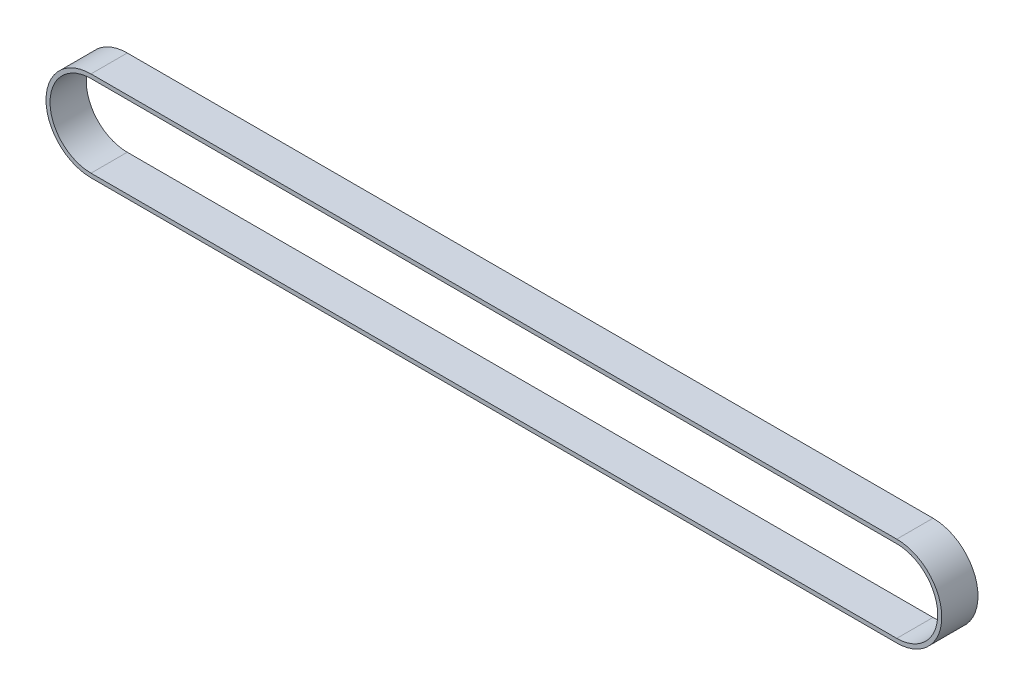
from build123d import *

# Parameters (mm, degrees)
BOSS_EXTRUDE1_DEPTH = 13.5


with BuildPart() as part:
    # Sketch1 → Boss-Extrude1 (new, symmetric)
    with BuildSketch(Plane.XY):
        with BuildLine():
            Line((0, 33.5), (600, 33.5))
            ThreePointArc((600, 33.5), (633.5, 0), (600, -33.5))
            Line((600, -33.5), (0, -33.5))
            ThreePointArc((0, -33.5), (-33.5, 0), (0, 33.5))
        make_face()
        with BuildLine():
            Line((0, 30.5), (600, 30.5))
            ThreePointArc((600, 30.5), (630.5, 0), (600, -30.5))
            Line((600, -30.5), (0, -30.5))
            ThreePointArc((0, -30.5), (-30.5, 0), (0, 30.5))
        make_face(mode=Mode.SUBTRACT)
    extrude(amount=BOSS_EXTRUDE1_DEPTH, both=True)


solid = part.part
